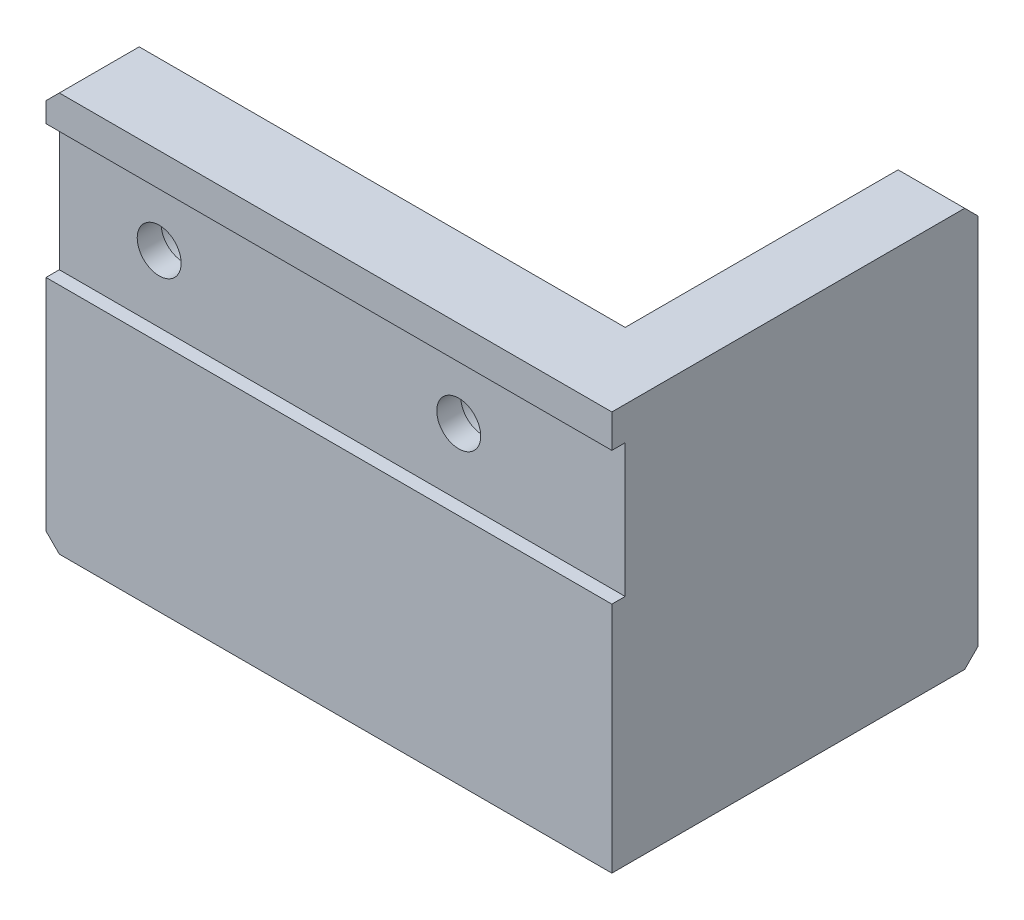
from build123d import *

# Parameters (mm, degrees)
SKETCH_2_W                   = 90
SKETCH_2_H                   = 60
EXTRUDE_1_DEPTH              = 12
SKETCH_3_W                   = 2
SKETCH_3_H                   = 20
CUT_EXTRUDE_1_DEPTH          = 109.830142883
SKETCH_4_W                   = 10
SKETCH_4_H                   = 1
CUT_EXTRUDE_2_DEPTH          = 109.830142883
HOLE_WIZARD_M6_3_D           = 6.6
HOLE_WIZARD_M6_3_DEPTH       = 17
HOLE_WIZARD_M6_3_CBORE_D     = 11
HOLE_WIZARD_M6_3_CBORE_DEPTH = 6.4
HOLE_WIZARD_M6_3_TIP         = 1.982840043
CHAMFER_1_SIZE               = 2
HOLE_WIZARD_M3_1_D           = 2.5
HOLE_WIZARD_M3_1_DEPTH       = 8.5
HOLE_WIZARD_M3_1_TIP         = 0.751075774
SKETCH_15_W                  = 10
SKETCH_15_H                  = 60
EXTRUDE_2_DEPTH              = 44
SKETCH_16_W                  = 5
SKETCH_16_H                  = 60
CUT_EXTRUDE_3_DEPTH          = 117.400171821
HOLE_WIZARD_M6_1_D           = 5
HOLE_WIZARD_M6_1_DEPTH       = 17
HOLE_WIZARD_M6_1_TIP         = 1.502151548
CHAMFER_2_SIZE               = 2


with BuildPart() as part:
    # 草图2 → 凸台-拉伸1 (new body)
    with BuildSketch(Plane.XY):
        with Locations((45, -30)):
            Rectangle(SKETCH_2_W, SKETCH_2_H)
    extrude(amount=EXTRUDE_1_DEPTH)

    # 草图3 → 切除-拉伸1 (cut, through all)
    with BuildSketch(Plane(origin=(90, 0, 0), x_dir=(0, 0, -1), z_dir=(1, 0, 0))):
        with Locations((-11, -15)):
            Rectangle(SKETCH_3_W, SKETCH_3_H)
    extrude(amount=-CUT_EXTRUDE_1_DEPTH, mode=Mode.SUBTRACT)

    # 草图4 → 切除-拉伸2 (cut, through all)
    with BuildSketch(Plane(origin=(0, 0, 0), x_dir=(1, 0, 0), z_dir=(0, 1, 0))):
        with Locations((80, -0.5)):
            Rectangle(SKETCH_4_W, SKETCH_4_H)
    extrude(amount=-CUT_EXTRUDE_2_DEPTH, mode=Mode.SUBTRACT)

    # M6 六角凹头螺钉的柱形沉头孔3
    with Locations(Plane(origin=(0, 0, 0), x_dir=(-1, 0, 0), z_dir=(0, 0, -1))):
        with Locations((-60, -15), (-15, -15)):
            CounterBoreHole(HOLE_WIZARD_M6_3_D / 2, HOLE_WIZARD_M6_3_CBORE_D / 2, HOLE_WIZARD_M6_3_CBORE_DEPTH, depth=HOLE_WIZARD_M6_3_DEPTH)
            with Locations((0, 0, -(HOLE_WIZARD_M6_3_DEPTH + HOLE_WIZARD_M6_3_TIP / 2))):  # 118° drill point
                Cone(0, HOLE_WIZARD_M6_3_D / 2, HOLE_WIZARD_M6_3_TIP, mode=Mode.SUBTRACT)

    # 倒角1
    chamfer_1_edges = [part.edges().sort_by_distance(p)[0] for p in [
        (0, 0, 6),
        (90, 0, 6),
        (90, -60, 6),
        (0, -60, 6),
    ]]
    chamfer(chamfer_1_edges, length=CHAMFER_1_SIZE)

    # M3 螺纹孔1
    with Locations(Plane(origin=(0, -60, 0), x_dir=(-1, 0, 0), z_dir=(0, -1, 0))):
        with Locations((-70, -6)):
            Hole(HOLE_WIZARD_M3_1_D / 2, depth=HOLE_WIZARD_M3_1_DEPTH)
            with Locations((0, 0, -(HOLE_WIZARD_M3_1_DEPTH + HOLE_WIZARD_M3_1_TIP / 2))):  # 118° drill point
                Cone(0, HOLE_WIZARD_M3_1_D / 2, HOLE_WIZARD_M3_1_TIP, mode=Mode.SUBTRACT)

    # 草图15 → 凸台-拉伸2 (add)
    with BuildSketch(Plane(origin=(0, 0, 1), x_dir=(-1, 0, 0), z_dir=(0, 0, -1))):
        with Locations((-80, -30)):
            Rectangle(SKETCH_15_W, SKETCH_15_H)
    extrude(amount=EXTRUDE_2_DEPTH)

    # 草图16 → 切除-拉伸3 (cut, through all)
    with BuildSketch(Plane(origin=(0, 0, 0), x_dir=(-1, 0, 0), z_dir=(0, 0, -1))):
        with Locations((-87.5, -30)):
            Rectangle(SKETCH_16_W, SKETCH_16_H)
    extrude(amount=-CUT_EXTRUDE_3_DEPTH, mode=Mode.SUBTRACT)

    # M6 螺纹孔1
    with Locations(Plane(origin=(0, 0, -43), x_dir=(-1, 0, 0), z_dir=(0, 0, -1))):
        with Locations((-80, -15), (-80, -45)):
            Hole(HOLE_WIZARD_M6_1_D / 2, depth=HOLE_WIZARD_M6_1_DEPTH)
            with Locations((0, 0, -(HOLE_WIZARD_M6_1_DEPTH + HOLE_WIZARD_M6_1_TIP / 2))):  # 118° drill point
                Cone(0, HOLE_WIZARD_M6_1_D / 2, HOLE_WIZARD_M6_1_TIP, mode=Mode.SUBTRACT)

    # 倒角2
    chamfer_2_edges = [part.edges().sort_by_distance(p)[0] for p in [
        (80, -60, -43),
        (80, 0, -43),
    ]]
    chamfer(chamfer_2_edges, length=CHAMFER_2_SIZE)


solid = part.part
